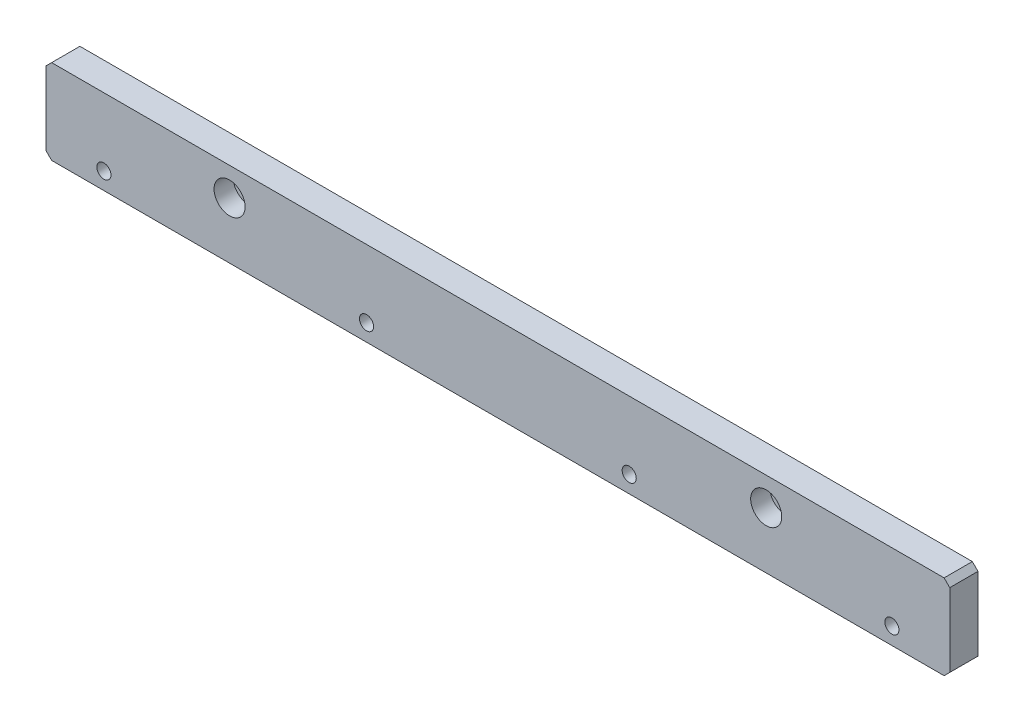
from build123d import *

# Parameters (mm, degrees)
SKETCH1_W           = 320
SKETCH1_H           = 30
BOSS_EXTRUDE1_DEPTH = 10
CHAMFER1_SIZE       = 2
M6_TAPPED_HOLE1_D   = 5
HOLE1_D             = 6.6
HOLE1_CBORE_D       = 11
HOLE1_CBORE_DEPTH   = 6.8


with BuildPart() as part:
    # Sketch1 → Boss-Extrude1 (new body)
    with BuildSketch(Plane.XY):
        Rectangle(SKETCH1_W, SKETCH1_H)
    extrude(amount=BOSS_EXTRUDE1_DEPTH)

    # Chamfer1
    chamfer1_edges = [part.edges().sort_by_distance(p)[0] for p in [
        (160, -15, 5),
        (-160, -15, 5),
        (-160, 15, 5),
        (160, 15, 5),
    ]]
    chamfer(chamfer1_edges, length=CHAMFER1_SIZE)

    # M6 Tapped Hole1 (through all)
    with Locations(Plane.XY.offset(10)):
        with Locations((-139.5, -9), (-46.5, -9), (46.5, -9), (139.5, -9)):
            Hole(M6_TAPPED_HOLE1_D / 2)

    # Hole1 (through all)
    with Locations(Plane.XY.offset(10)):
        with Locations((-95, 5), (95, 5)):
            CounterBoreHole(HOLE1_D / 2, HOLE1_CBORE_D / 2, HOLE1_CBORE_DEPTH)


solid = part.part
